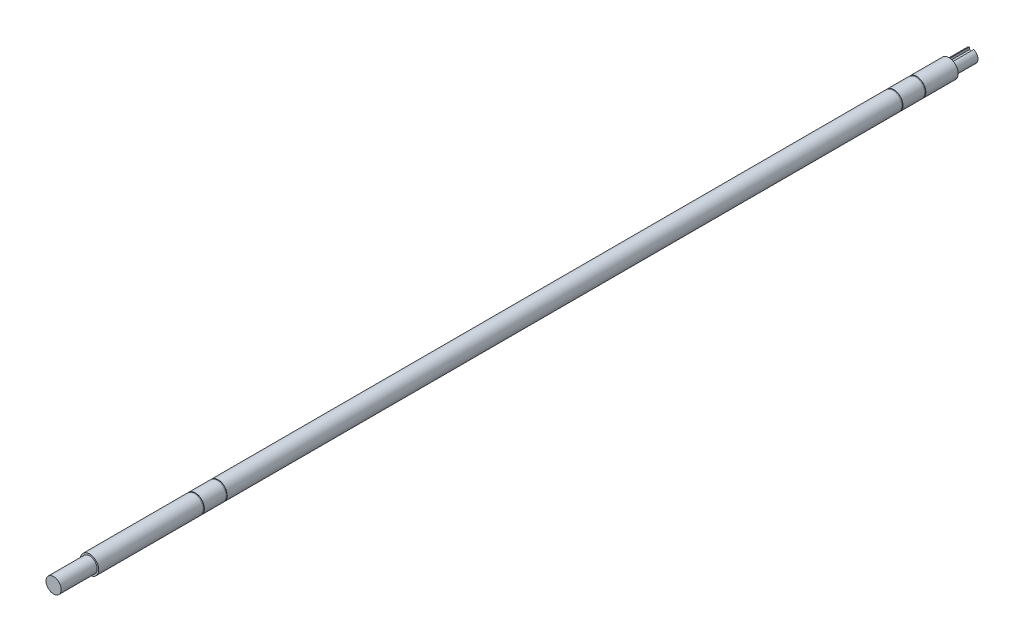
SolidWorks part; units mm, degrees
ref_plane "前视基准面" through (0, 0, 0) normal (0, 0, 1) x (1, 0, 0)
ref_plane "上视基准面" through (0, 0, 0) normal (0, 1, 0) x (1, 0, 0)
ref_plane "右视基准面" through (0, 0, 0) normal (1, 0, 0) x (0, 0, -1)
sketch "草图1" plane through (0, 0, 0) normal (0, 0, 1) x (1, 0, 0)
  circle A0 centre (0, 0) radius 7
  dimension "D1" = 14
extrude "凸台-拉伸1" add sketch "草图1" along normal mid plane 900
sketch "草图2" plane through (0, 0, 0) normal (0, 0, 1) x (1, 0, 0)
  circle A0 centre (0, 0) radius 8.5
  dimension "D1" = 17
extrude "凸台-拉伸2" add sketch "草图2" along normal mid plane 833.6
sketch "草图3" plane through (0, 0, -450) normal (0, 0, -1) x (-1, 0, 0)
  circle A0 centre (0, 0) radius 6
  circle A3 centre (0, 0) radius 8.5 construction
  circle A4 centre (0, 0) radius 8.5
  dimension "D1" = 12
extrude "切除-拉伸1" cut sketch "草图3" against normal up to surface (33.2 mm away) up to face at (7, 0, -416.8)
sketch "草图4" plane through (0, 0, 0) normal (0, 1, 0) x (1, 0, 0)
  line L0 (6, 450) -> (-6, 450) construction
  line L1 (-6, 450) -> (6, 450)
  line L2 (-6, 450) -> (-6, 437.55)
  line L3 (-6, 437.55) -> (6, 437.55)
  line L4 (6, 450) -> (6, 437.55)
  line L5 (6, 416.8) -> (6, 450) construction
  line L6 (-6, 450) -> (-6, 416.8) construction
  line L7 (0, 0) -> (197.0439, 0) construction
  dimension "D1" = 12.45
extrude "切除-拉伸2" cut sketch "草图4" against normal through all both and the other way through all
other "移动面1" face at (6, 0, -437.55) face at (8.5, 0, -416.8) parameters "D1"=40
sketch "草图21" plane through (0, 0, -397.55) normal (0, 0, -1) x (-1, 0, 0)
  line L0 (0, 0) -> (6, 0) construction
  line L1 (0, 0) -> (0, 6) construction
  circle A0 centre (0, 0) radius 6 construction
  circle A1 centre (0, 0) radius 6 construction
  dimension "D1" = 90
ref_plane "基准面1" through (0, 6, -397.55) normal (0, 1, 0) x (0, 0, 1)
sketch "草图31" plane through (0, 6, -397.55) normal (0, 1, 0) x (0, 0, 1)
  line L0 (-1, 0) -> (17.75, 0) construction
  line L1 (-1, 2) -> (17.75, 2)
  line L2 (-1, -2) -> (17.75, -2)
  line L3 (0, 0) -> (-1, 0) construction
  line L4 (0, 6) -> (0, -6) construction
  line L8 (20.75, 8.5) -> (20.75, -8.5) construction
  arc A0 (-1, 2) -> (-1, -2) centre (-1, 0) ccw
  arc A1 (17.75, -2) -> (17.75, 2) centre (17.75, 0) ccw
  point P2 (8.375, 0)
  dimension "D3" = 1
  dimension "D1" = 4
  dimension "D2" = 1
extrude "切除-拉伸11" cut sketch "草图31" against normal blind 2.5
sketch "草图34" plane through (0, 0, -397.55) normal (0, 0, -1) x (-1, 0, 0)
  point P0 (0, 0)
hole_wizard "M4 螺纹孔1" positions "草图34" profile "草图33" tap size "M4" standard "GB"
sketch "草图33" plane through (0, 0, -397.55) normal (1, 0, 0) x (0, 1, 0)
  line L0 (0, 0) -> (0, 11.0914)
  line L1 (0, 11.0914) -> (1.65, 10.1)
  line L2 (1.65, 10.1) -> (1.65, 0)
  line L5 (1.65, 0) -> (0, 0)
  line L10 (0, 11.0914) -> (-1.65, 10.1) construction
  line L11 (0, -6.35) -> (0, 107.95) construction
  dimension "螺纹孔钻头直径" = 3.3
  dimension "螺纹孔钻头深度" = 10.1
  dimension "导头角度" = 118
cosmetic thread "孔螺纹线1" parameters "D1"=8, "D2"=4
ref_plane "基准面2" through (0, 0, 319.2) normal (0, 0, 1) x (1, 0, 0)
sketch "草图35" plane through (0, 0, 319.2) normal (0, 0, 1) x (1, 0, 0)
  circle A0 centre (0, 0) radius 8.5 construction
  circle A1 centre (0, 0) radius 8.5
  circle A2 centre (0, 0) radius 8.1
  dimension "D1" = 16.2
extrude "切除-拉伸12" cut sketch "草图35" along normal blind 1.1
ref_plane "基准面3" through (0, 0, 298.1) normal (0, 0, 1) x (1, 0, 0)
sketch "草图36" plane through (0, 0, 298.1) normal (0, 0, 1) x (1, 0, 0)
  circle A0 centre (0, 0) radius 8.5 construction
  circle A1 centre (0, 0) radius 8.5
  circle A2 centre (0, 0) radius 8.1
  dimension "D1" = 16.2
extrude "切除-拉伸13" cut sketch "草图36" along normal blind 1.1
ref_plane "基准面4" through (0, 0, -325.8) normal (0, 0, 1) x (1, 0, 0)
sketch "草图37" plane through (0, 0, -325.8) normal (0, 0, 1) x (1, 0, 0)
  circle A0 centre (0, 0) radius 8.5 construction
  circle A1 centre (0, 0) radius 8.5
  circle A2 centre (0, 0) radius 8.1
  dimension "D1" = 16.2
extrude "切除-拉伸14" cut sketch "草图37" along normal blind 1.1
ref_plane "基准面5" through (0, 0, -346.9) normal (0, 0, 1) x (1, 0, 0)
sketch "草图38" plane through (0, 0, -346.9) normal (0, 0, 1) x (1, 0, 0)
  circle A0 centre (0, 0) radius 8.5 construction
  circle A1 centre (0, 0) radius 8.5
  circle A2 centre (0, 0) radius 8.1
  dimension "D1" = 16.2
extrude "切除-拉伸15" cut sketch "草图38" along normal blind 1.1
